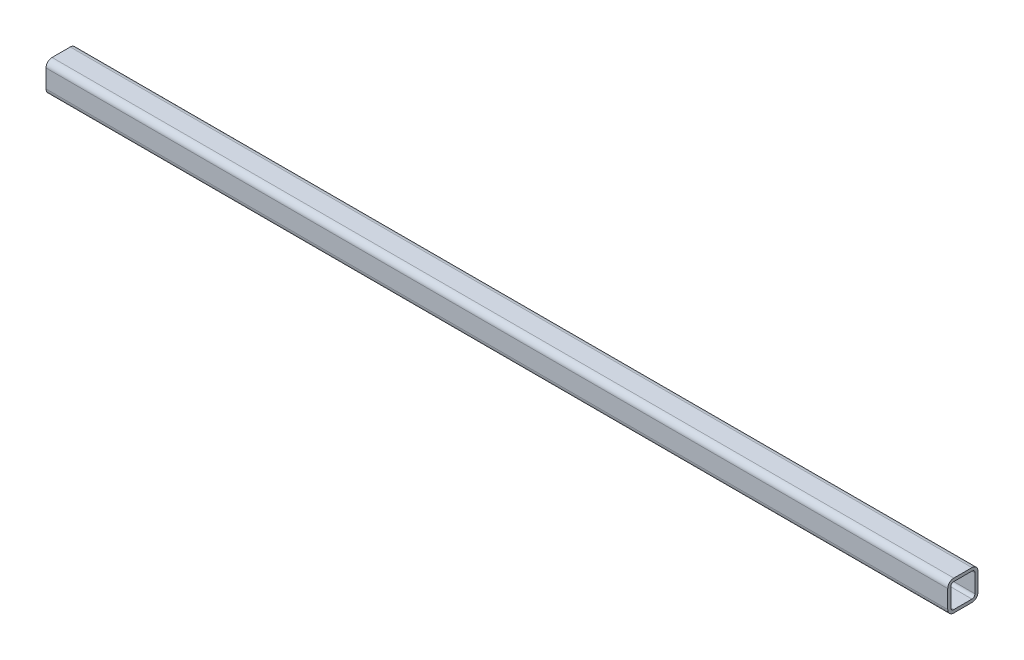
from build123d import *

# Parameters (mm, degrees)
SQUARE_TUBE_40_X_40_X_4_1_DEPTH = 1192


with BuildPart() as part:
    # Sketch1 → Square Tube 40 X 40 X 4(1) (new body)
    with BuildSketch(Plane.YZ.offset(-1000)):
        with BuildLine():
            Line((-12, -20), (12, -20))
            ThreePointArc((12, -20), (17.656854249, -17.656854249), (20, -12))
            Line((20, -12), (20, 12))
            ThreePointArc((20, 12), (17.656854249, 17.656854249), (12, 20))
            Line((12, 20), (-12, 20))
            ThreePointArc((-12, 20), (-17.656854249, 17.656854249), (-20, 12))
            Line((-20, 12), (-20, -12))
            ThreePointArc((-20, -12), (-17.656854249, -17.656854249), (-12, -20))
        make_face()
        with BuildLine():
            Line((-12, -16), (12, -16))
            ThreePointArc((12, -16), (14.828427125, -14.828427125), (16, -12))
            Line((16, -12), (16, 12))
            ThreePointArc((16, 12), (14.828427125, 14.828427125), (12, 16))
            Line((12, 16), (-12, 16))
            ThreePointArc((-12, 16), (-14.828427125, 14.828427125), (-16, 12))
            Line((-16, 12), (-16, -12))
            ThreePointArc((-16, -12), (-14.828427125, -14.828427125), (-12, -16))
        make_face(mode=Mode.SUBTRACT)
    extrude(amount=SQUARE_TUBE_40_X_40_X_4_1_DEPTH)


solid = part.part
